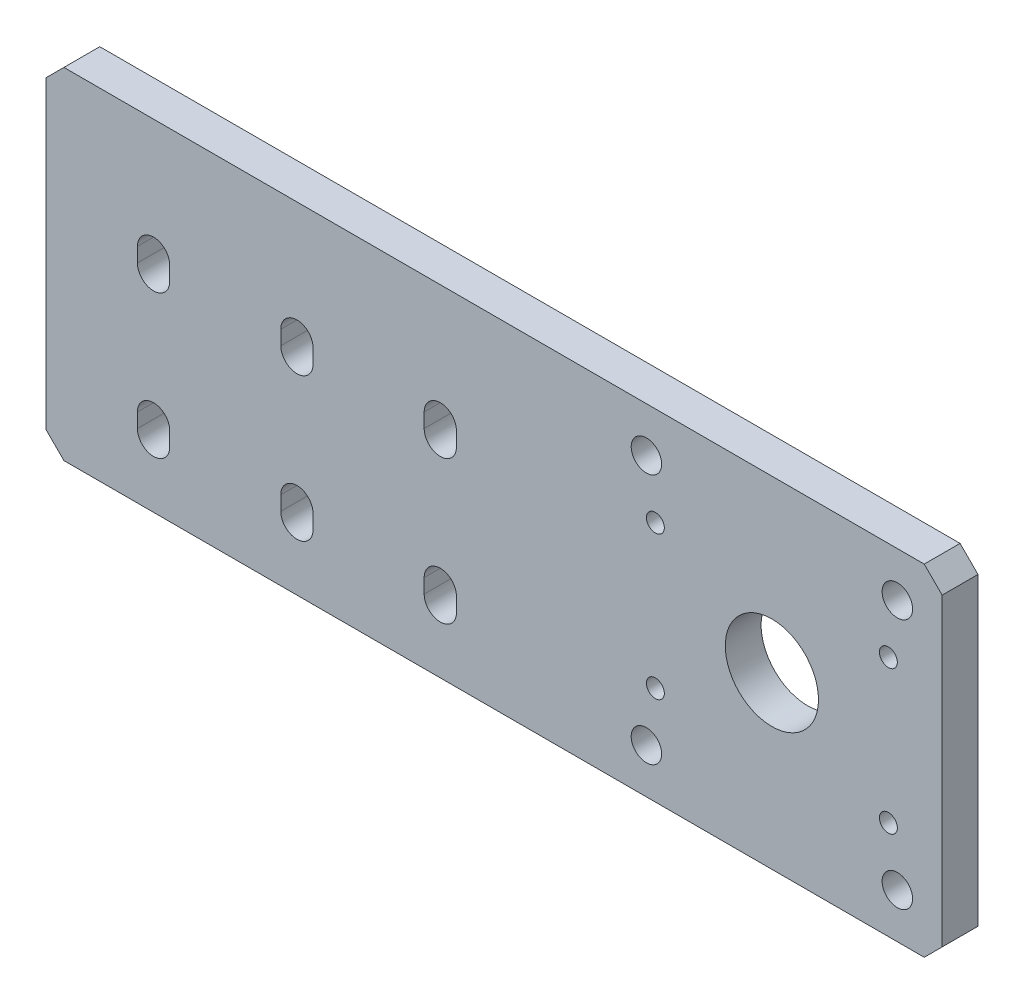
from build123d import *

# Parameters (mm, degrees)
SKETCH_1_W                  = 250
SKETCH_1_H                  = 95
EXTRUDE_1_DEPTH             = 10
CUT_EXTRUDE_2_DEPTH         = 135.094183319
PATTERN_LINEAR_1_COUNT      = 2
PATTERN_LINEAR_1_PITCH      = 40
PATTERN_LINEAR_1_COUNT_DIR2 = 2
PATTERN_LINEAR_1_PITCH_DIR2 = 40
PATTERN_LINEAR_2_COUNT      = 2
PATTERN_LINEAR_2_PITCH      = 40
PATTERN_LINEAR_2_COUNT_DIR2 = 2
PATTERN_LINEAR_2_PITCH_DIR2 = 40
CHAMFER_1_SIZE              = 5
HOLE_WIZARD_M10_3_D         = 8.5
HOLE_WIZARD_M10_3_DEPTH     = 24.5
HOLE_WIZARD_M10_3_TIP       = 2.553657631
SKETCH_12_R                 = 13
CUT_EXTRUDE_5_DEPTH         = 135.094183319
HOLE_WIZARD_M6_1_D          = 5
HOLE_WIZARD_M4_1_D          = 3.3
HOLE_WIZARD_M4_1_DEPTH      = 10.1
HOLE_WIZARD_M4_1_TIP        = 0.991420021


with BuildPart() as part:
    # 草图1 → 凸台-拉伸1 (new body)
    with BuildSketch(Plane.XY):
        Rectangle(SKETCH_1_W, SKETCH_1_H)
    extrude(amount=EXTRUDE_1_DEPTH)

    # 草图3 → 切除-拉伸2 (cut, through all)
    with BuildSketch(Plane.XY.offset(10)):
        with BuildLine():
            Line((-59.5, -29.5), (-59.5, -25.5))
            ThreePointArc((-59.5, -25.5), (-55, -21), (-50.5, -25.5))
            Line((-50.5, -25.5), (-50.5, -29.5))
            ThreePointArc((-50.5, -29.5), (-55, -34), (-59.5, -29.5))
        make_face()
    cut_extrude_2 = extrude(amount=-CUT_EXTRUDE_2_DEPTH, mode=Mode.SUBTRACT)

    # 阵列(线性)1: Cut-Extrude 2 2 × 2
    with Locations(*[(i * PATTERN_LINEAR_1_PITCH, j * PATTERN_LINEAR_1_PITCH_DIR2, 0) for i in range(PATTERN_LINEAR_1_COUNT) for j in range(PATTERN_LINEAR_1_COUNT_DIR2) if (i, j) != (0, 0)]):
        add(cut_extrude_2, mode=Mode.SUBTRACT)

    # 阵列(线性)2: Cut-Extrude 2 2 × 2
    with Locations(*[(-i * PATTERN_LINEAR_2_PITCH, j * PATTERN_LINEAR_2_PITCH_DIR2, 0) for i in range(PATTERN_LINEAR_2_COUNT) for j in range(PATTERN_LINEAR_2_COUNT_DIR2) if (i, j) != (0, 0)]):
        add(cut_extrude_2, mode=Mode.SUBTRACT)

    # 倒角1
    chamfer_1_edges = [part.edges().sort_by_distance(p)[0] for p in [
        (125, -47.5, 5),
        (-125, -47.5, 5),
        (-125, 47.5, 5),
        (125, 47.5, 5),
    ]]
    chamfer(chamfer_1_edges, length=CHAMFER_1_SIZE)

    # M10 螺纹孔3
    with Locations(Plane(origin=(42.5, 35, 10), x_dir=(1, 0, 0), z_dir=(0, 0, 1))):
        with Locations((0, 0), (70, 0), (70, -70), (0, -70)):
            Hole(HOLE_WIZARD_M10_3_D / 2, depth=HOLE_WIZARD_M10_3_DEPTH)
            with Locations((0, 0, -(HOLE_WIZARD_M10_3_DEPTH + HOLE_WIZARD_M10_3_TIP / 2))):  # 118° drill point
                Cone(0, HOLE_WIZARD_M10_3_D / 2, HOLE_WIZARD_M10_3_TIP, mode=Mode.SUBTRACT)

    # 草图12 → 切除-拉伸5 (cut, through all)
    with BuildSketch(Plane.XY.offset(10)):
        with Locations((77.5, 0)):
            Circle(SKETCH_12_R)
    extrude(amount=-CUT_EXTRUDE_5_DEPTH, mode=Mode.SUBTRACT)

    # M6 螺纹孔1 (through all)
    with Locations(Plane(origin=(45, -20, 0), x_dir=(-1, 0, 0), z_dir=(0, 0, -1))):
        with Locations((0, 0), (-65, 0), (-65, 40), (0, 40)):
            Hole(HOLE_WIZARD_M6_1_D / 2)

    # M4 螺纹孔1
    with Locations(Plane(origin=(117, -47.5, 5), x_dir=(0, 0, -1), z_dir=(0, -1, 0))):
        with Locations((0, 0), (0, -105), (0, -52.5)):
            Hole(HOLE_WIZARD_M4_1_D / 2, depth=HOLE_WIZARD_M4_1_DEPTH)
            with Locations((0, 0, -(HOLE_WIZARD_M4_1_DEPTH + HOLE_WIZARD_M4_1_TIP / 2))):  # 118° drill point
                Cone(0, HOLE_WIZARD_M4_1_D / 2, HOLE_WIZARD_M4_1_TIP, mode=Mode.SUBTRACT)


solid = part.part
